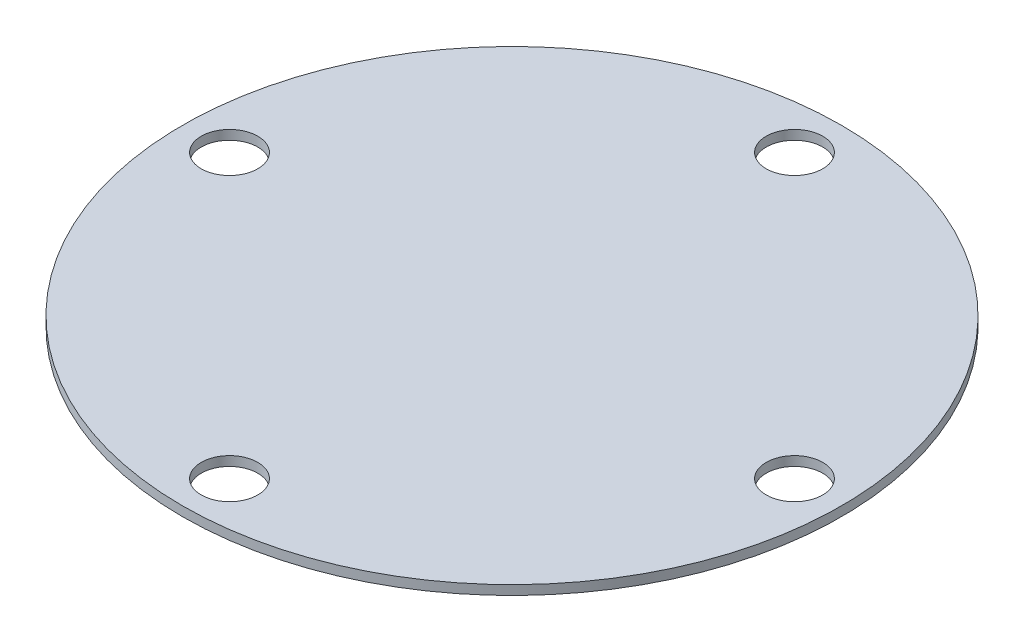
from build123d import *

# Parameters (mm, degrees)
SKETCH_1_R          = 70
EXTRUDE_1_DEPTH     = 2
SKETCH_3_R          = 6
CUT_EXTRUDE_1_DEPTH = 100.015150356


with BuildPart() as part:
    # 草图1 → 凸台-拉伸1 (new body)
    with BuildSketch(Plane(origin=(0, 0, 0), x_dir=(1, 0, 0), z_dir=(0, 1, 0))):
        with Locations(Location((0, 0, 0), (0, 0, 270))):
            Circle(SKETCH_1_R)
    extrude(amount=EXTRUDE_1_DEPTH)

    # 草图3 → 切除-拉伸1 (cut, through all)
    with BuildSketch(Plane(origin=(0, 2, 0), x_dir=(1, 0, 0), z_dir=(0, 1, 0))):
        with Locations(Location((0, 60, 0), (0, 0, 270))):
            Circle(SKETCH_3_R)
        with Locations(Location((60, 0, 0), (0, 0, 270))):
            Circle(SKETCH_3_R)
        with Locations(Location((0, -60, 0), (0, 0, 270))):
            Circle(SKETCH_3_R)
        with Locations(Location((-60, 0, 0), (0, 0, 270))):
            Circle(SKETCH_3_R)
    extrude(amount=-CUT_EXTRUDE_1_DEPTH, mode=Mode.SUBTRACT)


solid = part.part
